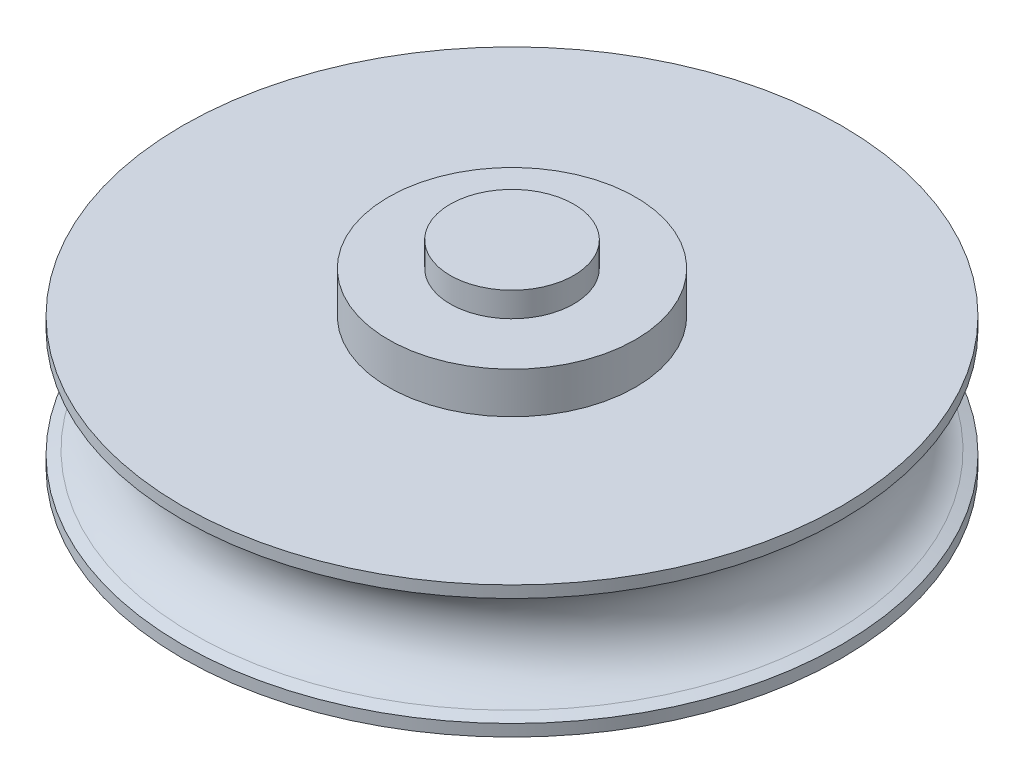
SolidWorks part; units mm, degrees
ref_plane "Front Plane" through (0, 0, 0) normal (0, 0, 1) x (1, 0, 0)
ref_plane "Top Plane" through (0, 0, 0) normal (0, 1, 0) x (1, 0, 0)
ref_plane "Right Plane" through (0, 0, 0) normal (1, 0, 0) x (0, 0, -1)
sketch "Sketch1" plane through (0, 0, 0) normal (0, 0, 1) x (1, 0, 0)
  line L0 (-15, 0) -> (-40, 0)
  line L1 (-40, 0) -> (-40, 1.4326)
  line L2 (-40, 1.4326) -> (-38.7162, 1.9144)
  line L3 (-38.7162, 14.0856) -> (-40, 14.5674)
  line L4 (-40, 14.5674) -> (-40, 16)
  line L5 (-40, 16) -> (-15, 16)
  line L6 (0, 24) -> (0, -8)
  line L7 (-15, 21) -> (-15, 16)
  line L8 (-15, -5) -> (-7.5, -5)
  line L9 (-7.5, -5) -> (-7.5, -8)
  line L10 (-7.5, -8) -> (0, -8)
  line L11 (-15, 0) -> (-15, -5)
  line L12 (-15, 21) -> (-7.5, 21)
  line L13 (-7.5, 21) -> (-7.5, 24)
  line L14 (-7.5, 24) -> (0, 24)
  arc A0 (-38.7162, 1.9144) -> (-38.7162, 14.0856) centre (-41, 8) ccw
  point P14 (-22.5, 8)
  dimension "D7" = 6.5
  dimension "D5" = 41
  dimension "D2" = 8
  dimension "D1" = 40
  dimension "D3" = 5
  dimension "D6" = 8
  dimension "D8" = 5
  dimension "D9" = 3
  dimension "D10" = 3
  dimension "D11" = 15
  dimension "D12" = 7.5
  dimension "D13" = 7.5
  dimension "D14" = 16
revolve "Revolve1" add sketch "Sketch1" angle 360 about L6
sketch "Sketch2" plane through (0, 0, 0) normal (0, -1, 0) x (-1, 0, 0)
  circle A0 centre (0, 0) radius 8
  dimension "D1" = 16
